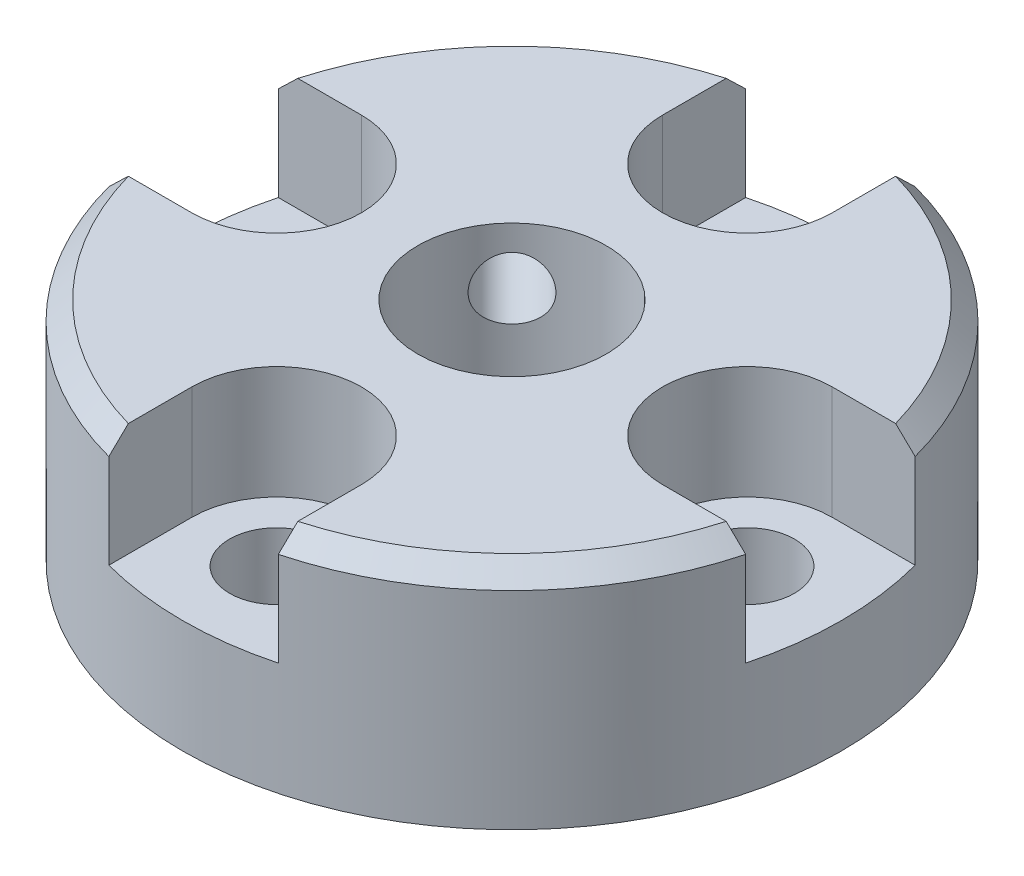
from build123d import *

# Parameters (mm, degrees)
SKETCH1_R                  = 17.5
SKETCH1_R_2                = 5
BOSS_EXTRUDE1_DEPTH        = 12
SKETCH4_R                  = 2.5
CUT_EXTRUDE2_DEPTH         = 28.504545079
SKETCH7_R                  = 4.5
CUT_EXTRUDE4_DEPTH         = 6
CUT_EXTRUDE5_DEPTH         = 6
CIRPATTERN1_COUNT          = 4
SKETCH9_W                  = 1.65
SKETCH9_H                  = 24.748737342
M4_TAPPED_HOLE1_AT_2_COUNT = 2
M4_TAPPED_HOLE1_AT_2_PITCH = 6
CHAMFER1_SIZE              = 1


with BuildPart() as part:
    # Sketch1 → Boss-Extrude1 (new body)
    with BuildSketch(Plane(origin=(0, 0, 0), x_dir=(1, 0, 0), z_dir=(0, 1, 0))):
        with Locations(Location((0, 0, 0), (0, 0, 270))):
            Circle(SKETCH1_R)
        with Locations(Location((0, 0, 0), (0, 0, 270))):
            Circle(SKETCH1_R_2, mode=Mode.SUBTRACT)
    extrude(amount=BOSS_EXTRUDE1_DEPTH)

    # Sketch4 → Cut-Extrude2 (cut, through all)
    with BuildSketch(Plane.XZ):
        with Locations(Location((0, 12.5, 0), (0, 0, 270))):
            Circle(SKETCH4_R)
        with Locations(Location((-12.5, 0, 0), (0, 0, 270))):
            Circle(SKETCH4_R)
        with Locations(Location((12.5, 0, 0), (0, 0, 270))):
            Circle(SKETCH4_R)
        with Locations(Location((0, -12.5, 0), (0, 0, 270))):
            Circle(SKETCH4_R)
    extrude(amount=-CUT_EXTRUDE2_DEPTH, mode=Mode.SUBTRACT)

    # Sketch7 → Cut-Extrude4 (cut)
    with BuildSketch(Plane(origin=(0, 12, 0), x_dir=(1, 0, 0), z_dir=(0, 1, 0))):
        with Locations(Location((0, 12.5, 0), (0, 0, 270))):
            Circle(SKETCH7_R)
        with Locations(Location((12.5, 0, 0), (0, 0, 270))):
            Circle(SKETCH7_R)
        with Locations(Location((0, -12.5, 0), (0, 0, 270))):
            Circle(SKETCH7_R)
        with Locations(Location((-12.5, 0, 0), (0, 0, 270))):
            Circle(SKETCH7_R)
    extrude(amount=-CUT_EXTRUDE4_DEPTH, mode=Mode.SUBTRACT)

    # Sketch8 → Cut-Extrude5 (cut)
    with BuildSketch(Plane(origin=(0, 12, 0), x_dir=(1, 0, 0), z_dir=(0, 1, 0))):
        with BuildLine():
            Line((-12.5, 4.5), (-21.528291401, 4.5))
            Line((-21.528291401, 4.5), (-21.528291401, -4.5))
            Line((-21.528291401, -4.5), (-12.5, -4.5))
            ThreePointArc((-12.5, -4.5), (-8, 0), (-12.5, 4.5))
        make_face()
    cut_extrude5 = extrude(amount=-CUT_EXTRUDE5_DEPTH, mode=Mode.SUBTRACT)

    # CirPattern1: Cut-Extrude5 ×4 about axis
    cirpattern1_axis = Axis((0, 0, 0), (0, 1, 0))
    for i in range(1, CIRPATTERN1_COUNT):
        add(cut_extrude5.rotate(cirpattern1_axis, i * 360 / CIRPATTERN1_COUNT), mode=Mode.SUBTRACT)

    # Sketch9 → M4 Tapped Hole1 (revolve, cut)
    with BuildSketch(Plane(origin=(0, 3, 0), x_dir=(0.7071067811865464, 0, -0.7071067811865488), z_dir=(0, 1, 0))):
        with Locations((0.825, 12.374368671)):
            Rectangle(SKETCH9_W, SKETCH9_H)
    m4_tapped_hole1 = revolve(axis=Axis((4.490128061, 3, 4.490128061), (-0.7071067811865487, 0, -0.7071067811865464)), mode=Mode.SUBTRACT)

    # M4 Tapped Hole1 at 2: M4 Tapped Hole1 ×2
    with Locations(*[(0, i * M4_TAPPED_HOLE1_AT_2_PITCH, 0) for i in range(1, M4_TAPPED_HOLE1_AT_2_COUNT)]):
        add(m4_tapped_hole1, mode=Mode.SUBTRACT)

    # Chamfer1
    chamfer1_edges = [part.edges().sort_by_distance(p)[0] for p in [
        (12.374368671, 12, 12.374368671),
        (-12.374368671, 12, 12.374368671),
        (-12.374368671, 12, -12.374368671),
        (12.374368671, 12, -12.374368671),
    ]]
    chamfer(chamfer1_edges, length=CHAMFER1_SIZE)


solid = part.part
